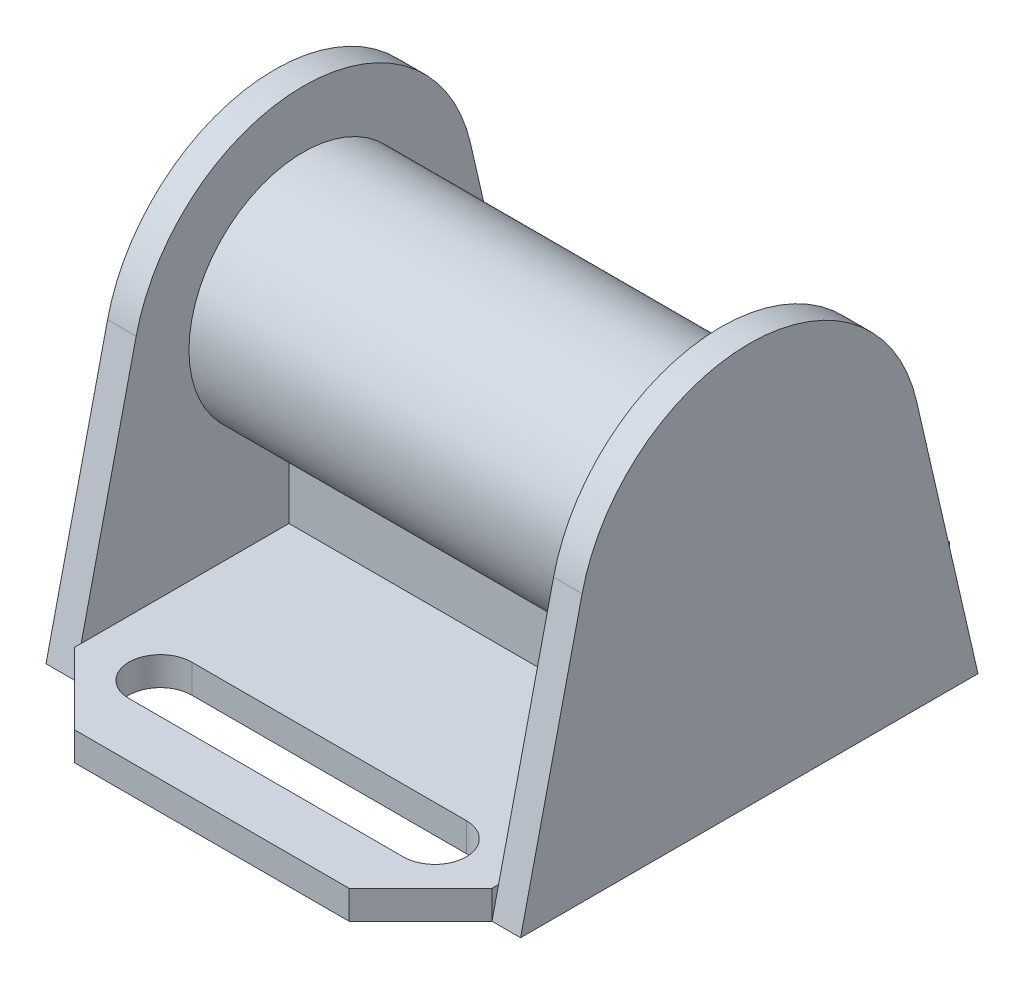
SolidWorks part; units mm, degrees
material "A3"
ref_plane "前视基准面" through (0, 0, 0) normal (0, 0, 1) x (1, 0, 0)
ref_plane "上视基准面" through (0, 0, 0) normal (0, 1, 0) x (1, 0, 0)
ref_plane "右视基准面" through (0, 0, 0) normal (1, 0, 0) x (0, 0, -1)
sketch "草图1" plane through (0, 0, 0) normal (0, 1, 0) x (1, 0, 0)
  line L0 (0, 0) -> (-73, 0) construction
  line L1 (-73, -80) -> (-73, 80)
  line L2 (-73, 80) -> (-48, 105)
  line L3 (-48, 105) -> (48, 105)
  line L4 (0, 105) -> (0, -105) construction
  line L5 (-48, 75) -> (48, 75) construction
  line L6 (-48, 86) -> (48, 86)
  line L7 (-48, 64) -> (48, 64)
  line L8 (73, -80) -> (73, 80)
  line L9 (73, 80) -> (48, 105)
  line L10 (-48, -75) -> (48, -75) construction
  line L11 (-48, -86) -> (48, -86)
  line L12 (-48, -64) -> (48, -64)
  line L13 (73, -80) -> (48, -105)
  line L14 (-48, -105) -> (48, -105)
  line L15 (-73, -80) -> (-48, -105)
  arc A0 (-48, 86) -> (-48, 64) centre (-48, 75) ccw
  arc A1 (48, 64) -> (48, 86) centre (48, 75) ccw
  arc A2 (-48, -86) -> (-48, -64) centre (-48, -75) cw
  arc A3 (48, -64) -> (48, -86) centre (48, -75) cw
  point P8 (0, 75)
  point P20 (0, -75)
  point P28 (73, 0)
  dimension "D6" = 25
  dimension "D1" = 160
  dimension "D2" = 210
  dimension "D3" = 25
  dimension "D4" = 146
  dimension "D5" = 22
  dimension "D7" = 75
extrude "凸台-拉伸1" add sketch "草图1" along normal blind 10
sketch "草图2" plane through (-73, 0, 0) normal (-1, 0, 0) x (0, 0, 1)
  line L0 (-80, 0) -> (-58.4687, 93.4687)
  line L1 (0, 80) -> (0, 0) construction
  line L2 (80, 0) -> (58.4687, 93.4687)
  line L3 (-80, 0) -> (80, 0)
  arc A0 (58.4687, 93.4687) -> (-58.4687, 93.4687) centre (0, 80) ccw
  dimension "D1" = 120
  dimension "D2" = 80
extrude "凸台-拉伸2" add sketch "草图2" along normal blind 10 separate body
mirror "镜向1" about plane through (0, 0, 0) normal (1, 0, 0) of bodies 107
sketch "草图3" plane through (0, 0, 0) normal (1, 0, 0) x (0, 0, -1)
  circle A0 centre (0, 80) radius 32
  circle A1 centre (0, 80) radius 40
  dimension "D1" = 64
  dimension "D2" = 80
extrude "凸台-拉伸3" add sketch "草图3" along normal up to next (73 mm away) and the other way up to next (73 mm away) separate body
sketch "草图4" plane through (0, 10, 0) normal (0, 1, 0) x (1, 0, 0)
  line L0 (73, 58.4687) -> (73, -58.4687) construction
  line L1 (-73, 5) -> (73, 5)
  line L2 (-73, 5) -> (-73, -5)
  line L3 (-73, -5) -> (73, -5)
  line L4 (73, 5) -> (73, -5)
  line L5 (-73, 5) -> (73, -5) construction
  line L6 (-73, -5) -> (73, 5) construction
  point P0 (0, 0)
  dimension "D1" = 10
extrude "凸台-拉伸4" add sketch "草图4" along normal up to body separate body
